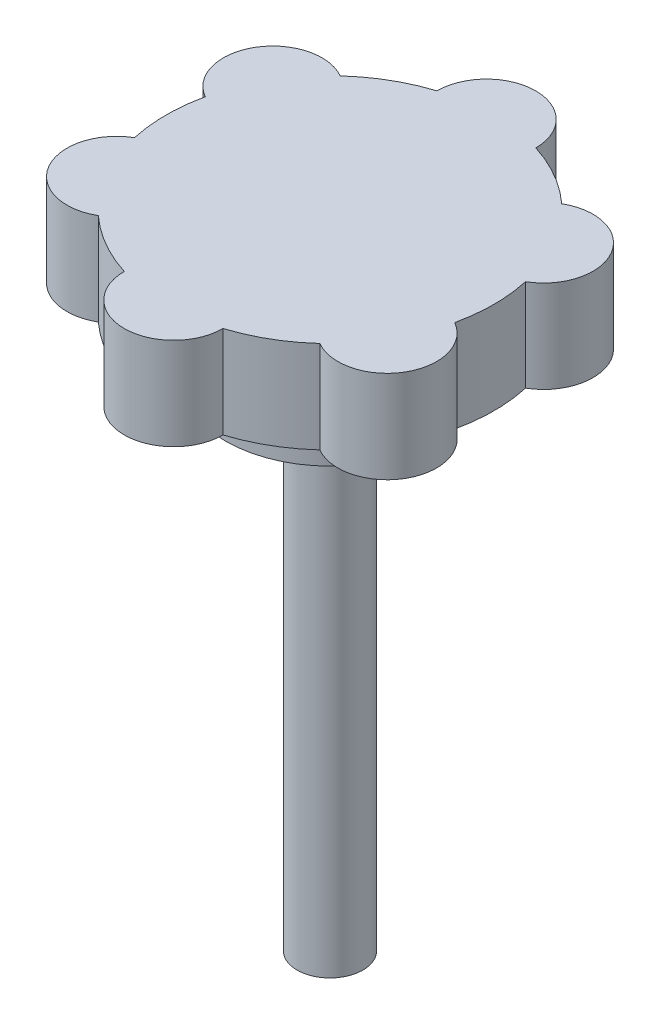
SolidWorks part; units mm, degrees
ref_plane "Front Plane" through (0, 0, 0) normal (0, 0, 1) x (1, 0, 0)
ref_plane "Top Plane" through (0, 0, 0) normal (0, 1, 0) x (1, 0, 0)
ref_plane "Right Plane" through (0, 0, 0) normal (1, 0, 0) x (0, 0, -1)
sketch "Sketch1" plane through (0, 0, 0) normal (0, 1, 0) x (1, 0, 0)
  line L21 (-6.7261, 7.3469) -> (-6.7267, 7.3472)
  line L22 (-3, 9.4991) -> (-3, 9.5)
  line L23 (6.7272, 7.3486) -> (6.7277, 7.3489)
  line L24 (-9.7242, -2.1519) -> (-9.7257, -2.1528)
  line L25 (-9.725, 2.1501) -> (-9.7267, 2.1511)
  line L26 (-2.998, -9.498) -> (-2.998, -9.5)
  line L27 (-6.7234, -7.3476) -> (-6.7257, -7.3489)
  line L28 (6.7276, -7.3465) -> (6.7287, -7.3472)
  line L29 (3.002, -9.4976) -> (3.002, -9.5)
  line L30 (9.7275, 2.1526) -> (9.7277, 2.1528)
  line L31 (9.7276, -2.1504) -> (9.7287, -2.1511)
  arc A2 (3, 9.5) -> (-3, 9.5) centre (0, 9.5) ccw
  arc A4 (9.7277, 2.1528) -> (6.7277, 7.3489) centre (8.2277, 4.7509) ccw
  arc A6 (6.7287, -7.3472) -> (9.7287, -2.1511) centre (8.2287, -4.7491) ccw
  arc A8 (-2.998, -9.5) -> (3.002, -9.5) centre (0.002, -9.5) ccw
  arc A10 (-9.7257, -2.1528) -> (-6.7257, -7.3489) centre (-8.2257, -4.7509) ccw
  arc A12 (-6.7267, 7.3472) -> (-9.7267, 2.1511) centre (-8.2267, 4.7491) ccw
  arc A13 (-9.725, 2.1501) -> (-9.7242, -2.1519) centre (0.0015, 0.0009) ccw
  arc A17 (-3, 9.4991) -> (-6.7261, 7.3469) centre (0.0015, 0.0009) ccw
  arc A18 (6.7272, 7.3486) -> (3, 9.5) centre (0.0015, 0.0009) ccw
  arc A22 (-6.7234, -7.3476) -> (-2.998, -9.498) centre (0.0015, 0.0009) ccw
  arc A25 (3.002, -9.4976) -> (6.7276, -7.3465) centre (0.0015, 0.0009) ccw
  arc A26 (9.7276, -2.1504) -> (9.7275, 2.1526) centre (0.0015, 0.0009) ccw
  point P53 (-4.1131, 2.3741)
  dimension "D2" = 3
extrude "Boss-Extrude1" add sketch "Sketch1" along normal blind 5.6
sketch "Sketch2" plane through (0, 0, 0) normal (0, -1, 0) x (1, 0, 0)
  circle A0 centre (0, 0) radius 6.35
  dimension "D1" = 12.7
extrude "Boss-Extrude2" add sketch "Sketch2" along normal blind 3.4
sketch "Sketch3" plane through (0, -3.4, 0) normal (0, -1, 0) x (1, 0, 0)
  circle A0 centre (0, 0) radius 2
  dimension "D1" = 4
extrude "Boss-Extrude3" add sketch "Sketch3" along normal blind 30
